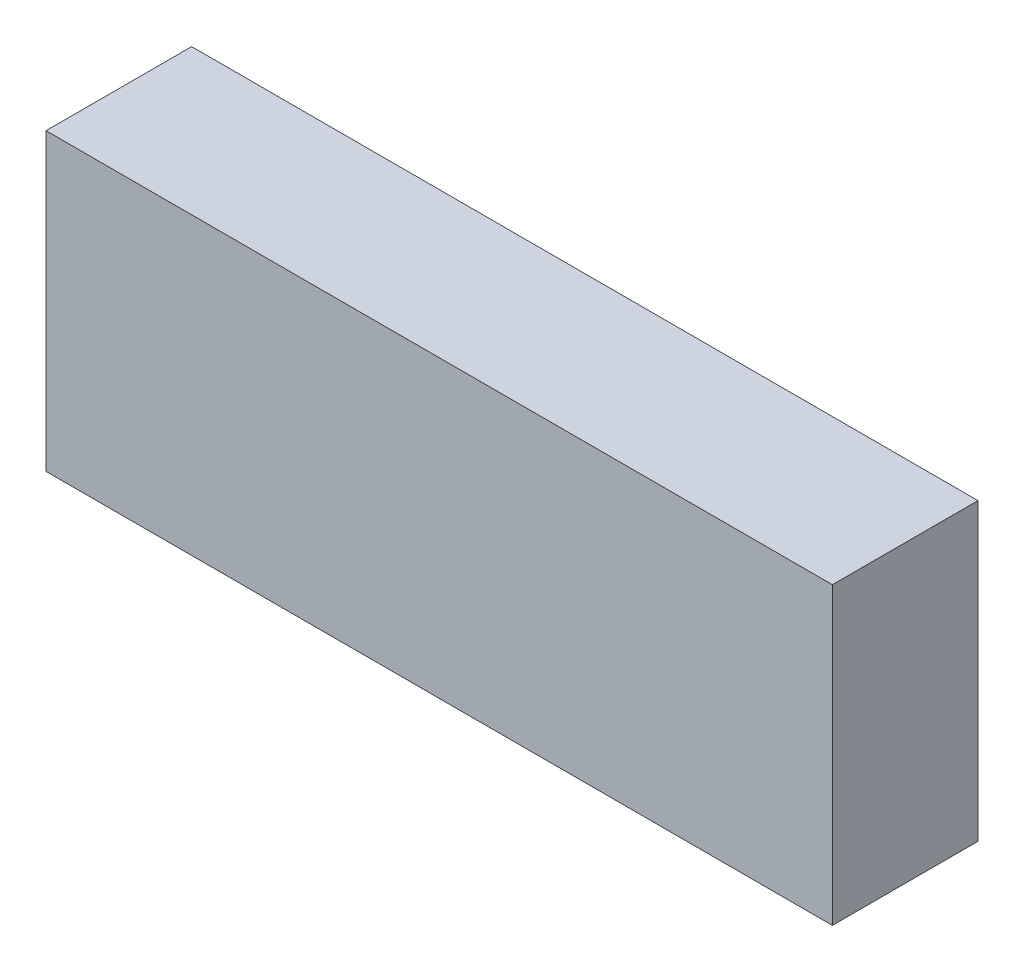
from build123d import *

# Parameters (mm, degrees)
SKETCH2_W           = 250
SKETCH2_H           = 93.801020924
BOSS_EXTRUDE1_DEPTH = 44
MOVE_FACE1_BY       = 2.3


with BuildPart() as part:
    # Sketch2 → Boss-Extrude1 (new body)
    with BuildSketch(Plane.XY):
        with Locations((0, 780.701531386)):
            Rectangle(SKETCH2_W, SKETCH2_H)
    extrude(amount=BOSS_EXTRUDE1_DEPTH)

    # Move Face1: a face moved outward by 2.3
    extrude(part.faces().sort_by_distance((0, 780.701531386, 44))[0], amount=MOVE_FACE1_BY, dir=(0, 0, 1))


solid = part.part
